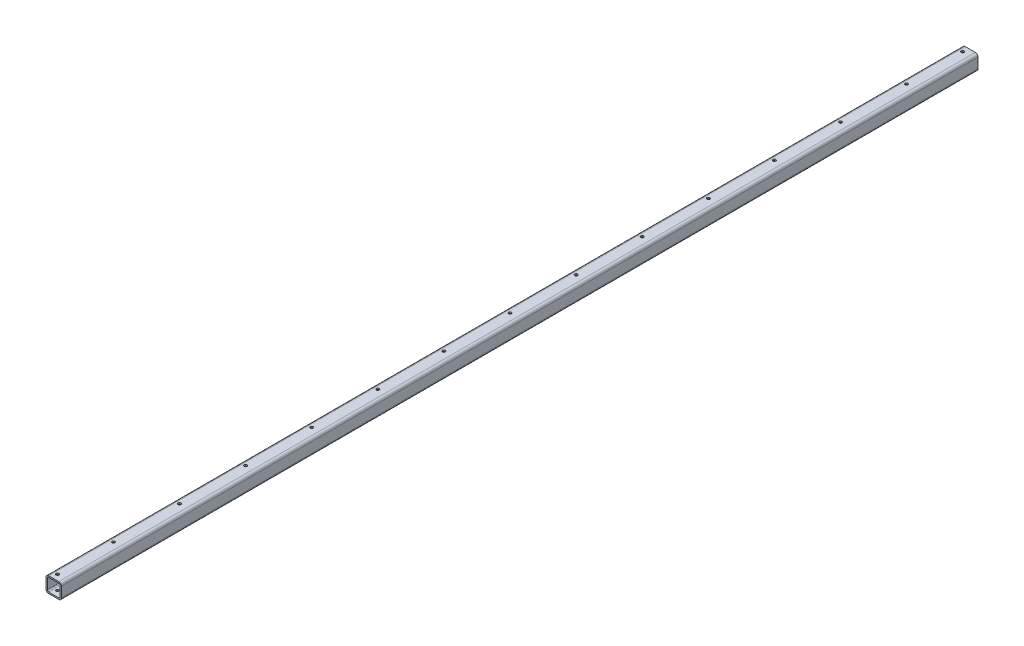
from build123d import *

# Parameters (mm, degrees)
BOSS_EXTRUDE1_DEPTH = 4160
SKETCH2_R           = 6.5
CUT_EXTRUDE1_DEPTH  = 4162.177717906
SKETCH3_R           = 6.5
CUT_EXTRUDE2_DEPTH  = 4162.177717906


with BuildPart() as part:
    # Sketch1 → Boss-Extrude1 (new body)
    with BuildSketch(Plane.XY):
        with BuildLine():
            Line((12, 0), (58, 0))
            ThreePointArc((58, 0), (66.485281374, 3.514718626), (70, 12))
            Line((70, 12), (70, 58))
            ThreePointArc((70, 58), (66.485281374, 66.485281374), (58, 70))
            Line((58, 70), (12, 70))
            ThreePointArc((12, 70), (3.514718626, 66.485281374), (0, 58))
            Line((0, 58), (0, 12))
            ThreePointArc((0, 12), (3.514718626, 3.514718626), (12, 0))
        make_face()
        with BuildLine():
            Line((12, 6), (58, 6))
            ThreePointArc((58, 6), (62.242640687, 7.757359313), (64, 12))
            Line((64, 12), (64, 58))
            ThreePointArc((64, 58), (62.242640687, 62.242640687), (58, 64))
            Line((58, 64), (12, 64))
            ThreePointArc((12, 64), (7.757359313, 62.242640687), (6, 58))
            Line((6, 58), (6, 12))
            ThreePointArc((6, 12), (7.757359313, 7.757359313), (12, 6))
        make_face(mode=Mode.SUBTRACT)
    extrude(amount=BOSS_EXTRUDE1_DEPTH)

    # Sketch2 → Cut-Extrude1 (cut, through all)
    with BuildSketch(Plane(origin=(0, 70, 0), x_dir=(1, 0, 0), z_dir=(0, 1, 0))):
        with Locations(Location((26, -280, 0), (0, 0, 270))):
            Circle(SKETCH2_R)
        with Locations(Location((26, -580, 0), (0, 0, 270))):
            Circle(SKETCH2_R)
        with Locations(Location((26, -880, 0), (0, 0, 270))):
            Circle(SKETCH2_R)
        with Locations(Location((26, -1180, 0), (0, 0, 270))):
            Circle(SKETCH2_R)
        with Locations(Location((26, -1480, 0), (0, 0, 270))):
            Circle(SKETCH2_R)
        with Locations(Location((26, -1780, 0), (0, 0, 270))):
            Circle(SKETCH2_R)
        with Locations(Location((26, -2080, 0), (0, 0, 270))):
            Circle(SKETCH2_R)
        with Locations(Location((26, -2380, 0), (0, 0, 270))):
            Circle(SKETCH2_R)
        with Locations(Location((26, -2680, 0), (0, 0, 270))):
            Circle(SKETCH2_R)
        with Locations(Location((26, -2980, 0), (0, 0, 270))):
            Circle(SKETCH2_R)
        with Locations(Location((26, -3280, 0), (0, 0, 270))):
            Circle(SKETCH2_R)
        with Locations(Location((26, -3580, 0), (0, 0, 270))):
            Circle(SKETCH2_R)
        with Locations(Location((26, -3880, 0), (0, 0, 270))):
            Circle(SKETCH2_R)
    extrude(amount=-CUT_EXTRUDE1_DEPTH, mode=Mode.SUBTRACT)

    # Sketch3 → Cut-Extrude2 (cut, through all)
    with BuildSketch(Plane(origin=(0, 70, 0), x_dir=(1, 0, 0), z_dir=(0, 1, 0))):
        with Locations(Location((26, -26, 0), (0, 0, 270))):
            Circle(SKETCH3_R)
        with Locations(Location((26, -4134, 0), (0, 0, 270))):
            Circle(SKETCH3_R)
    extrude(amount=-CUT_EXTRUDE2_DEPTH, mode=Mode.SUBTRACT)


solid = part.part
